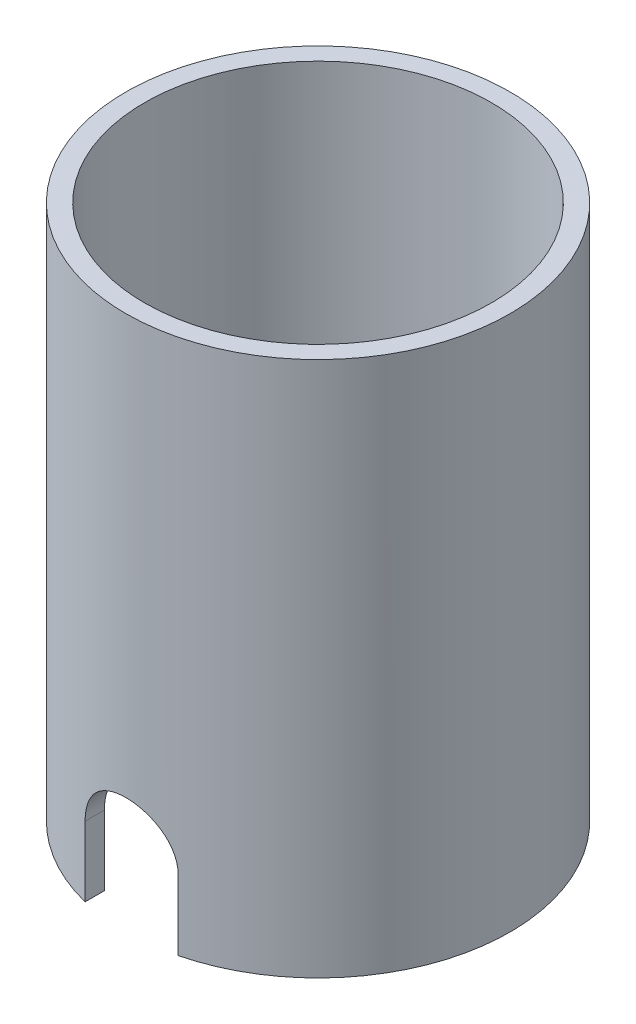
SolidWorks part; units mm, degrees
material "Q235B"
ref_plane "Front Plane" through (0, 0, 0) normal (0, 0, 1) x (1, 0, 0)
ref_plane "Top Plane" through (0, 0, 0) normal (0, 1, 0) x (1, 0, 0)
ref_plane "Right Plane" through (0, 0, 0) normal (1, 0, 0) x (0, 0, -1)
sketch "Sketch1" plane through (0, 0, 0) normal (0, 1, 0) x (1, 0, 0)
  circle A0 centre (0, 0) radius 82.5
  circle A1 centre (0, 0) radius 74.5
  dimension "D1" = 165
  dimension "D2" = 8
extrude "Boss-Extrude1" add sketch "Sketch1" along normal blind 230
sketch "Sketch2" plane through (0, 0, 0) normal (0, 0, 1) x (1, 0, 0)
  line L0 (0, 0) -> (0, 30) construction
  line L1 (-82.5, 0) -> (82.5, 0) construction
  line L2 (-20, 0) -> (-20, 30)
  line L3 (20, 0) -> (20, 30)
  arc A0 (-20, 0) -> (20, 0) centre (0, 0) ccw
  arc A1 (20, 30) -> (-20, 30) centre (0, 30) ccw
  point P4 (0, 15)
  dimension "D2" = 20
  dimension "D1" = 30
extrude "Cut-Extrude1" cut sketch "Sketch2" along normal up to next
